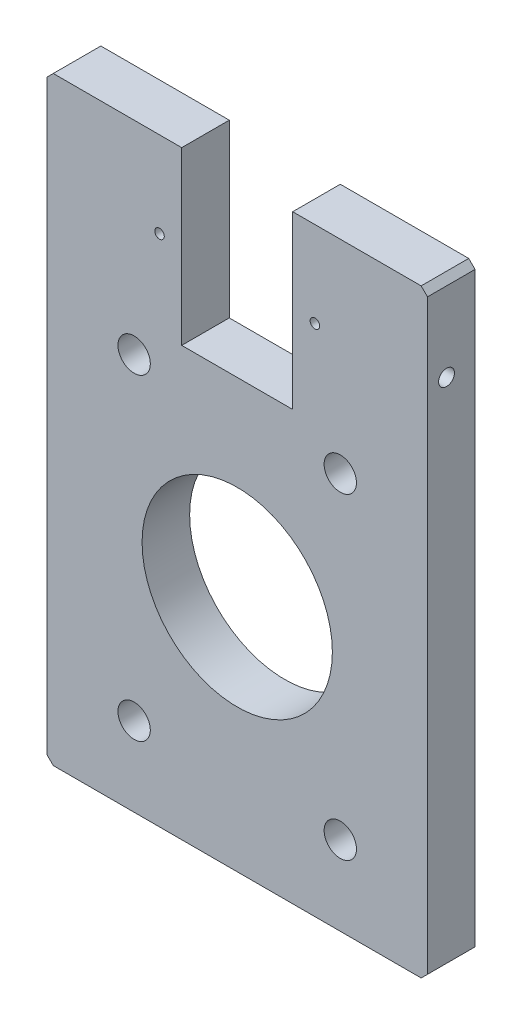
from build123d import *

# Parameters (mm, degrees)
SKETCH1_R                  = 5.1
BOSS_EXTRUDE1_DEPTH        = 15
SIZE_MM_DOWEL_HOLE_1_D     = 3
SIZE_MM_DOWEL_HOLE_1_DEPTH = 39.098709071
SIZE_MM_DOWEL_HOLE_1_TIP   = 0.901290929
SIZE_MM_DOWEL_HOLE_2_D     = 3
SIZE_MM_DOWEL_HOLE_2_DEPTH = 40
SIZE_MM_DOWEL_HOLE_2_TIP   = 0.901290929
M6_TAPPED_HOLE2_D          = 5
M6_TAPPED_HOLE2_DEPTH      = 17
M6_TAPPED_HOLE2_TIP        = 1.502151548
M12_TAPPED_HOLE1_D         = 10.2
SKETCH26_R                 = 30
CUT_EXTRUDE8_DEPTH         = 20
SIZE_MM_DOWEL_HOLE_3_D     = 3
SIZE_MM_DOWEL_HOLE_3_DEPTH = 19.75
SIZE_MM_DOWEL_HOLE_3_TIP   = 0.901290929
SKETCH28_R                 = 1.5
BOSS_EXTRUDE2_DEPTH        = 7
BOSS_EXTRUDE2_2_DEPTH      = 7


with BuildPart() as part:
    # Sketch1 → Boss-Extrude1 (new body)
    with BuildSketch(Plane.XY):
        Polygon((17.5, 94.5), (58, 94.5), (60, 92.5), (60, -92.5), (58, -94.5), (-58, -94.5), (-60, -92.5), (-60, 92.5), (-58, 94.5), (-17.5, 94.5), (-17.5, 40.5), (17.5, 40.5), align=None)
        with Locations((-32.5, -69.5)):
            Circle(SKETCH1_R, mode=Mode.SUBTRACT)
        with Locations((-32.5, 30.5)):
            Circle(SKETCH1_R, mode=Mode.SUBTRACT)
        with Locations((32.5, 30.5)):
            Circle(SKETCH1_R, mode=Mode.SUBTRACT)
        with Locations((32.5, -69.5)):
            Circle(SKETCH1_R, mode=Mode.SUBTRACT)
    extrude(amount=BOSS_EXTRUDE1_DEPTH)

    # Size mm dowel hole 1
    with Locations(Plane(origin=(60, 67.5, 9), x_dir=(0, 1, 0), z_dir=(1, 0, 0))):
        with Locations((0, 0)):
            Hole(SIZE_MM_DOWEL_HOLE_1_D / 2, depth=SIZE_MM_DOWEL_HOLE_1_DEPTH)
            with Locations((0, 0, -(SIZE_MM_DOWEL_HOLE_1_DEPTH + SIZE_MM_DOWEL_HOLE_1_TIP / 2))):  # 118° drill point
                Cone(0, SIZE_MM_DOWEL_HOLE_1_D / 2, SIZE_MM_DOWEL_HOLE_1_TIP, mode=Mode.SUBTRACT)

    # Size mm dowel hole 2
    with Locations(Plane(origin=(-60, 67.5, 9), x_dir=(0, -1, 0), z_dir=(-1, 0, 0))):
        with Locations((0, 0)):
            Hole(SIZE_MM_DOWEL_HOLE_2_D / 2, depth=SIZE_MM_DOWEL_HOLE_2_DEPTH)
            with Locations((0, 0, -(SIZE_MM_DOWEL_HOLE_2_DEPTH + SIZE_MM_DOWEL_HOLE_2_TIP / 2))):  # 118° drill point
                Cone(0, SIZE_MM_DOWEL_HOLE_2_D / 2, SIZE_MM_DOWEL_HOLE_2_TIP, mode=Mode.SUBTRACT)

    # Sketch22 → M6 Tapped Hole1 (revolve, cut)
    with BuildSketch(Plane(origin=(-60, 67.5, 9), x_dir=(0, 0, 1), z_dir=(0, 1, 0))):
        Polygon((0, 0), (0, 18.502151548), (2.5, 17), (2.5, 0), align=None)
    revolve(axis=Axis((-66.35, 67.5, 9), (1, 0, 0)), mode=Mode.SUBTRACT)

    # M6 Tapped Hole2
    with Locations(Plane(origin=(60, 67.5, 9), x_dir=(0, 1, 0), z_dir=(1, 0, 0))):
        with Locations((0, 0)):
            Hole(M6_TAPPED_HOLE2_D / 2, depth=M6_TAPPED_HOLE2_DEPTH)
            with Locations((0, 0, -(M6_TAPPED_HOLE2_DEPTH + M6_TAPPED_HOLE2_TIP / 2))):  # 118° drill point
                Cone(0, M6_TAPPED_HOLE2_D / 2, M6_TAPPED_HOLE2_TIP, mode=Mode.SUBTRACT)

    # M12 Tapped Hole1 (through all)
    with Locations(Plane(origin=(-32.5, 30.5, 15), x_dir=(1, 0, 0), z_dir=(0, 0, 1))):
        with Locations((0, 0), (65, 0), (65, -100), (0, -100)):
            Hole(M12_TAPPED_HOLE1_D / 2)

    # Sketch26 → Cut-Extrude8 (cut)
    with BuildSketch(Plane.XY.offset(15)):
        with Locations((0, -19.5)):
            Circle(SKETCH26_R)
    extrude(amount=-CUT_EXTRUDE8_DEPTH, mode=Mode.SUBTRACT)

    # Size mm dowel hole 3
    with Locations(Plane(origin=(-24.5, 67.5, 15), x_dir=(1, 0, 0), z_dir=(0, 0, 1))):
        with Locations((0, 0), (49, 0)):
            Hole(SIZE_MM_DOWEL_HOLE_3_D / 2, depth=SIZE_MM_DOWEL_HOLE_3_DEPTH)
            with Locations((0, 0, -(SIZE_MM_DOWEL_HOLE_3_DEPTH + SIZE_MM_DOWEL_HOLE_3_TIP / 2))):  # 118° drill point
                Cone(0, SIZE_MM_DOWEL_HOLE_3_D / 2, SIZE_MM_DOWEL_HOLE_3_TIP, mode=Mode.SUBTRACT)


with BuildPart() as body_2:
    # Sketch28 → Boss-Extrude2 (new body)
    with BuildSketch(Plane(origin=(0, 0, 0), x_dir=(-1, 0, 0), z_dir=(0, 0, -1))):
        with Locations((24.5, 67.5)):
            Circle(SKETCH28_R)
    extrude(amount=-BOSS_EXTRUDE2_DEPTH)


with BuildPart() as body_3:
    # Sketch28 → Boss-Extrude2 2 (new body)
    with BuildSketch(Plane(origin=(0, 0, 0), x_dir=(-1, 0, 0), z_dir=(0, 0, -1))):
        with Locations((-24.5, 67.5)):
            Circle(SKETCH28_R)
    extrude(amount=-BOSS_EXTRUDE2_2_DEPTH)


solid = Compound([part.part, body_2.part, body_3.part])
